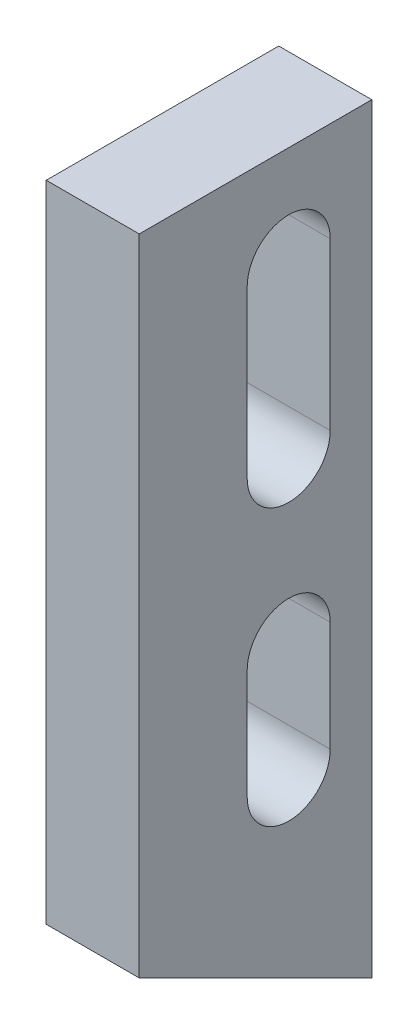
from build123d import *

# Parameters (mm, degrees)
BOSS_EXTRUDE1_DEPTH = 20
CHAMFER1_SIZE       = 12


with BuildPart() as part:
    # Sketch1 → Boss-Extrude1 (new, symmetric)
    with BuildSketch(Plane(origin=(0, 0, 0), x_dir=(0, 0, -1), z_dir=(1, 0, 0))):
        Polygon((0, 0), (70, -35), (70, 194), (0, 194), align=None)
        with BuildLine():
            Line((32.5, 114), (32.5, 164))
            ThreePointArc((32.5, 164), (45, 176.5), (57.5, 164))
            Line((57.5, 164), (57.5, 114))
            ThreePointArc((57.5, 114), (45, 101.5), (32.5, 114))
        make_face(mode=Mode.SUBTRACT)
        with BuildLine():
            Line((32.5, 30.910324642), (32.5, 64))
            ThreePointArc((32.5, 64), (45, 76.5), (57.5, 64))
            Line((57.5, 64), (57.5, 30.910324642))
            ThreePointArc((57.5, 30.910324642), (45, 18.410324642), (32.5, 30.910324642))
        make_face(mode=Mode.SUBTRACT)
    extrude(amount=BOSS_EXTRUDE1_DEPTH, both=True)

    # Chamfer1
    chamfer1_edges = [part.edges().sort_by_distance(p)[0] for p in [
        (-20, 194, -35),
        (-20, 79.5, -70),
        (-20, -17.5, -35),
        (-20, 97, 0),
    ]]
    chamfer(chamfer1_edges, length=CHAMFER1_SIZE)


solid = part.part
